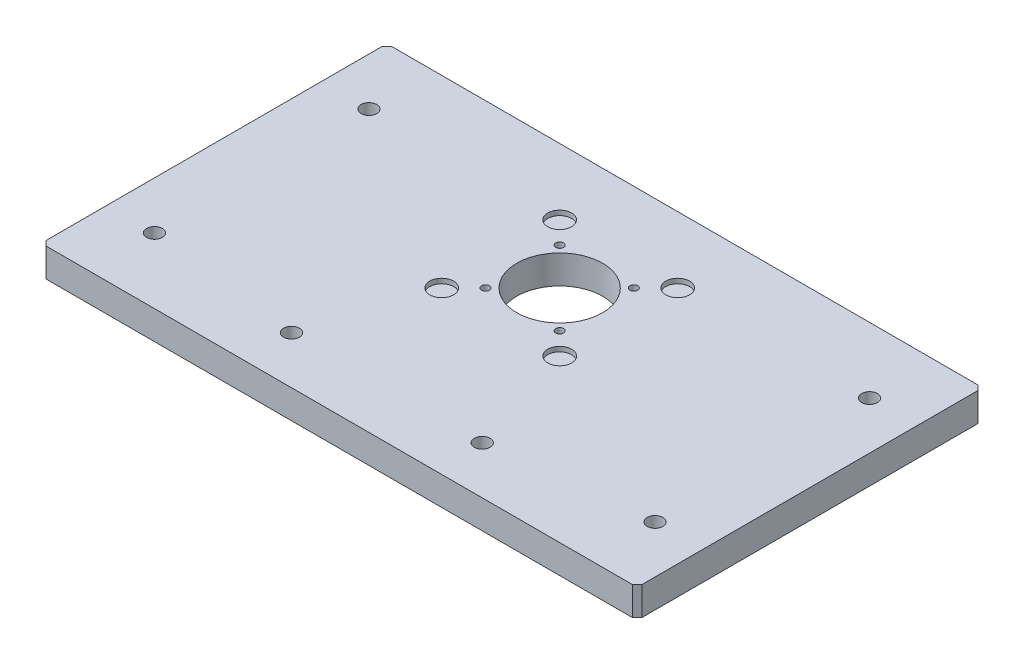
from build123d import *

# Parameters (mm, degrees)
SKETCH_1_W                   = 250
SKETCH_1_H                   = 145
EXTRUDE_1_DEPTH              = 12
CHAMFER_1_SIZE               = 2
SKETCH_2_R                   = 18
CUT_EXTRUDE_1_DEPTH          = 146.000862066
HOLE_WIZARD_M4_1_D           = 3.3
HOLE_WIZARD_M6_1_D           = 6.6
HOLE_WIZARD_M6_1_CBORE_D     = 11
HOLE_WIZARD_M6_1_CBORE_DEPTH = 6.8
SKETCH_11_R                  = 5
CUT_EXTRUDE_2_DEPTH          = 2


with BuildPart() as part:
    # 草图1 → 凸台-拉伸1 (new body)
    with BuildSketch(Plane(origin=(0, 0, 0), x_dir=(1, 0, 0), z_dir=(0, 1, 0))):
        Rectangle(SKETCH_1_W, SKETCH_1_H)
    extrude(amount=EXTRUDE_1_DEPTH)

    # 倒角1
    chamfer_1_edges = [part.edges().sort_by_distance(p)[0] for p in [
        (125, 6, 72.5),
        (-125, 6, 72.5),
        (-125, 6, -72.5),
        (125, 6, -72.5),
    ]]
    chamfer(chamfer_1_edges, length=CHAMFER_1_SIZE)

    # 草图2 → 切除-拉伸1 (cut, through all)
    with BuildSketch(Plane(origin=(0, 12, 0), x_dir=(1, 0, 0), z_dir=(0, 1, 0))):
        with Locations(Location((0, 20, 0), (0, 0, 270))):
            Circle(SKETCH_2_R)
    extrude(amount=-CUT_EXTRUDE_1_DEPTH, mode=Mode.SUBTRACT)

    # M4 螺纹孔1 (through all)
    with Locations(Plane(origin=(0, 0, 0), x_dir=(-1, 0, 0), z_dir=(0, -1, 0))):
        with Locations((15.556349186, 35.556349186), (-15.556349186, 35.556349186), (-15.556349186, 4.443650814), (15.556349186, 4.443650814)):
            Hole(HOLE_WIZARD_M4_1_D / 2)

    # M6 六角圆柱头螺钉的柱形沉头孔1 (through all)
    with Locations(Plane(origin=(0, 0, 0), x_dir=(-1, 0, 0), z_dir=(0, -1, 0))):
        with Locations((-40, -52.5), (-105, 45), (-105, -45), (105, 45), (105, -45), (40, -52.5)):
            CounterBoreHole(HOLE_WIZARD_M6_1_D / 2, HOLE_WIZARD_M6_1_CBORE_D / 2, HOLE_WIZARD_M6_1_CBORE_DEPTH)

    # 草图11 → 切除-拉伸2 (cut)
    with BuildSketch(Plane(origin=(0, 12, 0), x_dir=(1, 0, 0), z_dir=(0, 1, 0))):
        with Locations(Location((24.748737342, -4.748737342, 0), (0, 0, 270))):
            Circle(SKETCH_11_R)
        with Locations(Location((-24.748737342, -4.748737342, 0), (0, 0, 270))):
            Circle(SKETCH_11_R)
        with Locations(Location((-24.748737342, 44.748737342, 0), (0, 0, 270))):
            Circle(SKETCH_11_R)
        with Locations(Location((24.748737342, 44.748737342, 0), (0, 0, 270))):
            Circle(SKETCH_11_R)
    extrude(amount=-CUT_EXTRUDE_2_DEPTH, mode=Mode.SUBTRACT)


solid = part.part
